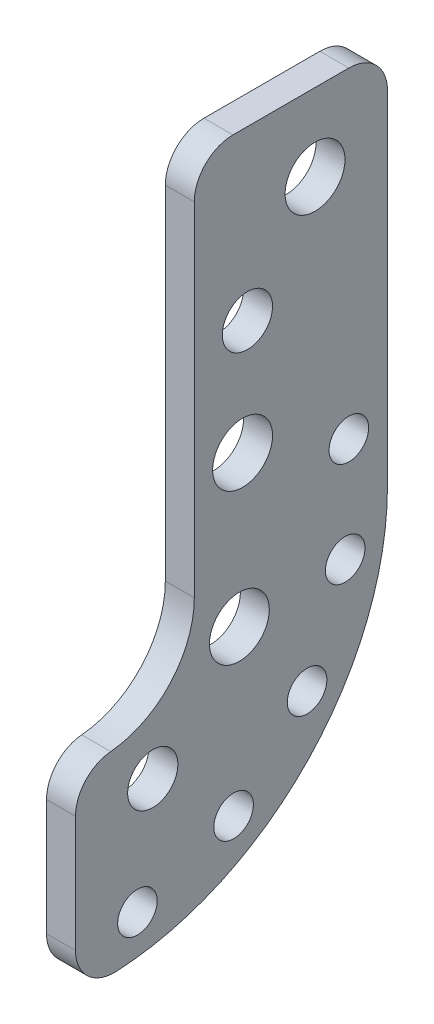
from build123d import *

# Parameters (mm, degrees)
SKETCH_1_R      = 1.025
SKETCH_1_R_2    = 1.3
SKETCH_1_R_3    = 1.55
EXTRUDE_1_DEPTH = 1.5
FILLET_R2_1_R   = 2


with BuildPart() as part:
    # 草图1 → 凸台-拉伸1 (new body)
    with BuildSketch(Plane(origin=(0, 0, 0), x_dir=(0, 0, -1), z_dir=(1, 0, 0))):
        with BuildLine():
            Line((-9.25, 0), (-9.25, 19.75))
            Line((-9.25, 19.75), (-19.25, 19.75))
            Line((-19.25, 19.75), (-19.25, 0))
            ThreePointArc((-19.25, 0), (-20.641242789, -3.358757211), (-24, -4.75))
            Line((-24, -4.75), (-25.4, -4.75))
            Line((-25.4, -4.75), (-25.4, -14.75))
            Line((-25.4, -14.75), (-24, -14.75))
            ThreePointArc((-24, -14.75), (-13.570174977, -10.429825023), (-9.25, 0))
        make_face()
        with Locations((-11.438131953, -2.182194118)):
            Circle(SKETCH_1_R, mode=Mode.SUBTRACT)
        with Locations((-13.411740816, -7.102905565)):
            Circle(SKETCH_1_R, mode=Mode.SUBTRACT)
        with Locations((-17.216155884, -10.795460111)):
            Circle(SKETCH_1_R, mode=Mode.SUBTRACT)
        with Locations((-22.193559229, -12.621381531)):
            Circle(SKETCH_1_R, mode=Mode.SUBTRACT)
        with Locations((-11.25, 3.116215025)):
            Circle(SKETCH_1_R, mode=Mode.SUBTRACT)
        with Locations((-21.4, -7.034912935)):
            Circle(SKETCH_1_R_2, mode=Mode.SUBTRACT)
        with Locations((-16.917350474, -2.466997302)):
            Circle(SKETCH_1_R_3, mode=Mode.SUBTRACT)
        with Locations((-16.75, 5.25)):
            Circle(SKETCH_1_R_3, mode=Mode.SUBTRACT)
        with Locations((-13, 15.75)):
            Circle(SKETCH_1_R_3, mode=Mode.SUBTRACT)
        with Locations((-16.5, 11.05)):
            Circle(SKETCH_1_R_2, mode=Mode.SUBTRACT)
    extrude(amount=EXTRUDE_1_DEPTH)

    # R2 圆角1
    fillet_r2_1_edges = [part.edges().sort_by_distance(p)[0] for p in [
        (0.75, 19.75, 19.25),
        (0.75, 19.75, 9.25),
        (0.75, -4.75, 25.4),
        (0.75, -14.75, 25.4),
    ]]
    fillet(fillet_r2_1_edges, radius=FILLET_R2_1_R)


solid = part.part
